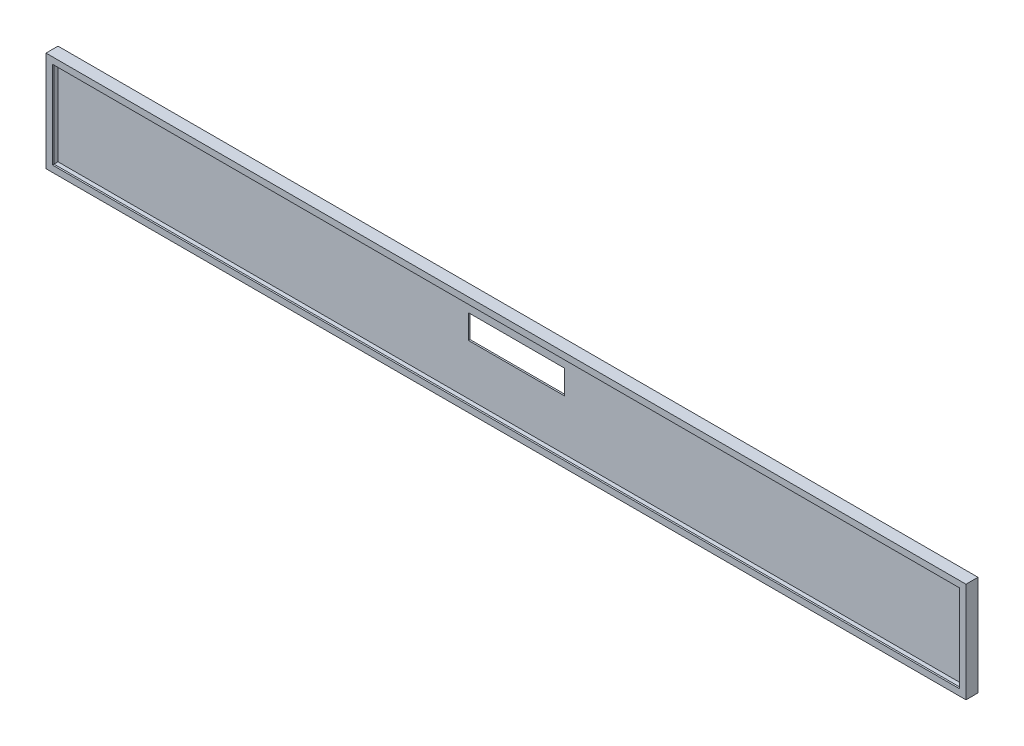
SolidWorks part; units mm, degrees
ref_plane "前视基准面" through (0, 0, 0) normal (0, 0, 1) x (1, 0, 0)
ref_plane "上视基准面" through (0, 0, 0) normal (0, 1, 0) x (1, 0, 0)
ref_plane "右视基准面" through (0, 0, 0) normal (1, 0, 0) x (0, 0, -1)
sketch "草图1" plane through (0, 0, 0) normal (0, 0, 1) x (1, 0, 0)
  line L1 (0, 0) -> (1148, 0)
  line L2 (0, 0) -> (0, 125)
  line L3 (0, 125) -> (1148, 125)
  line L4 (1148, 0) -> (1148, 125)
  dimension "D1" = 125
  dimension "D2" = 1148
extrude "凸台-拉伸1" add sketch "草图1" along normal blind 15
shell "抽壳1" thickness 2
sketch "草图2" plane through (0, 0, 15) normal (0, 0, 1) x (1, 0, 0)
  line L0 (8, 117) -> (8, 8)
  line L1 (0, 125) -> (1148, 125)
  line L2 (0, 125) -> (0, 0)
  line L3 (0, 0) -> (1148, 0)
  line L4 (1148, 125) -> (1148, 0)
  line L5 (8, 8) -> (1140, 8)
  line L6 (1140, 117) -> (1140, 8)
  line L7 (8, 117) -> (1140, 117)
  dimension "D1" = 8
extrude "凸台-拉伸2" add sketch "草图2" against normal blind 2
sketch "草图3" plane through (0, 0, 0) normal (0, 0, -1) x (-1, 0, 0)
  line L0 (-574, 125) -> (-574, -144.4869) construction
  line L1 (-634, 95) -> (-514, 95)
  line L2 (-634, 95) -> (-634, 65)
  line L3 (-634, 65) -> (-514, 65)
  line L4 (-514, 95) -> (-514, 65)
  line L5 (-1148, 125) -> (0, 125) construction
  dimension "D1" = 120
  dimension "D2" = 60
  dimension "D3" = 30
  dimension "D4" = 30
extrude "切除-拉伸1" cut sketch "草图3" against normal blind 10
